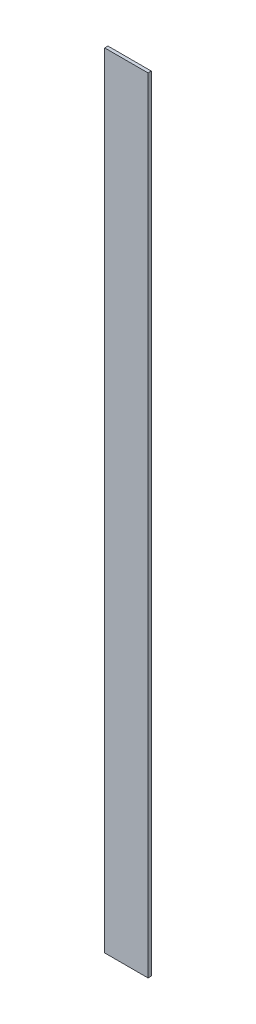
SolidWorks part; units mm, degrees
material "普通碳钢"
ref_plane "Front Plane" through (0, 0, 0) normal (0, 0, 1) x (1, 0, 0)
ref_plane "Top Plane" through (0, 0, 0) normal (0, 1, 0) x (1, 0, 0)
ref_plane "Right Plane" through (0, 0, 0) normal (1, 0, 0) x (0, 0, -1)
sketch "Sketch1" plane through (0, 0, 0) normal (0, 0, 1) x (1, 0, 0)
  line L1 (-200, 3613) -> (200, 3613)
  line L2 (-200, 3613) -> (-200, -3613)
  line L3 (-200, -3613) -> (200, -3613)
  line L4 (200, 3613) -> (200, -3613)
  dimension "D1" = 7226
  dimension "D2" = 400
  dimension "D3" = 3613
  dimension "D4" = 200
extrude "Boss-Extrude1" add sketch "Sketch1" along normal mid plane 30
